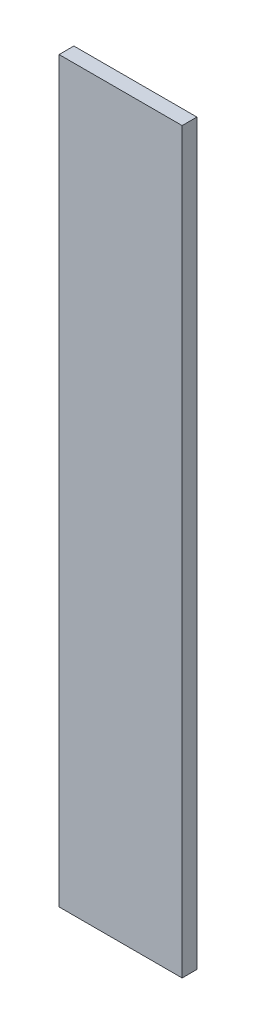
from build123d import *

# Parameters (mm, degrees)
SKETCH_1_W      = 25
SKETCH_1_H      = 150
EXTRUDE_1_DEPTH = 1.5


with BuildPart() as part:
    # 草图1 → 凸台-拉伸1 (new, symmetric)
    with BuildSketch(Plane.XY):
        Rectangle(SKETCH_1_W, SKETCH_1_H)
    extrude(amount=EXTRUDE_1_DEPTH, both=True)


solid = part.part
